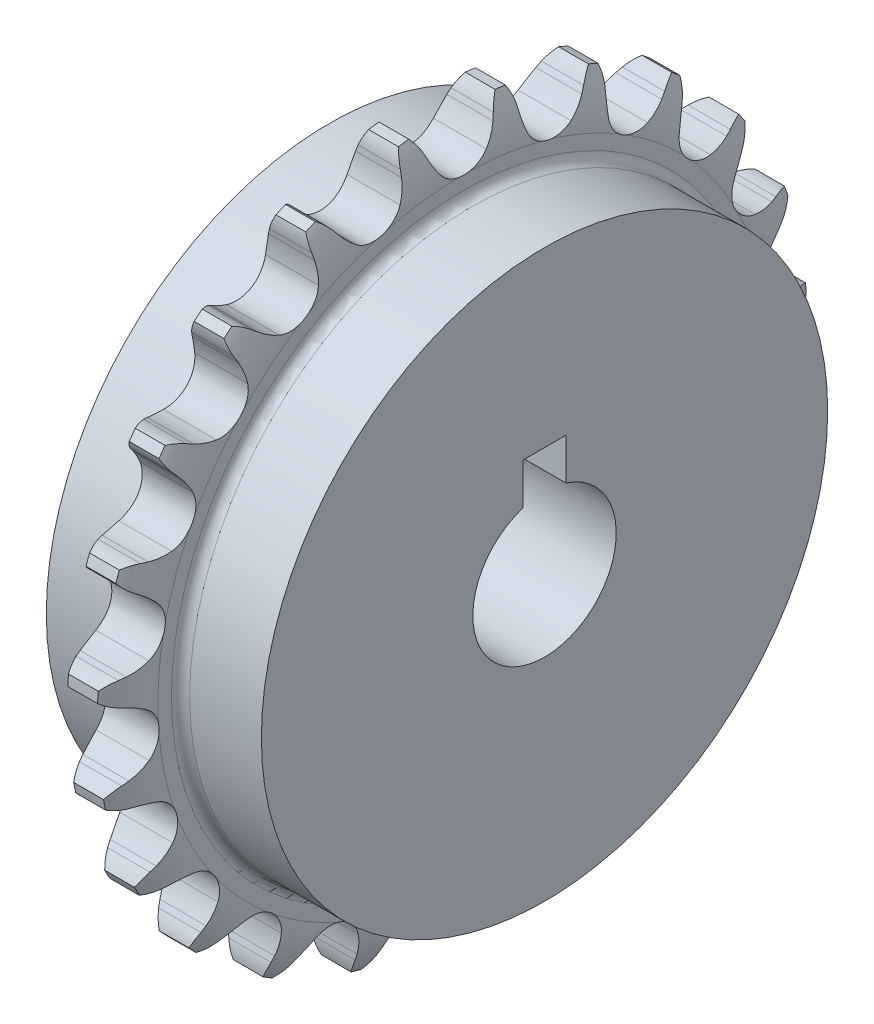
from build123d import *

# Parameters (mm, degrees)
EXTRUDECUTONE_DEPTH      = 5.315766473
PATTERNONE_COUNT         = 23
SKETCH_1_2_R             = 39.5
EXTRUDE_1_DEPTH          = 15
CUT_EXTRUDE_B_DEPTH      = 72.543477978
CUT_EXTRUDE_B_DEPTH_BACK = 72.543477978


with BuildPart() as part:
    # Sketch 1 → Revolve 2 (revolve)
    with BuildSketch(Plane.XY, mode=Mode.PRIVATE) as revolve_2_sk:
        with BuildLine():
            Line((-5.315766473, 0), (-5.315766473, 39.5))
            Line((-5.315766473, 39.5), (-4.998363178, 39.5))
            ThreePointArc((-4.998363178, 39.5), (-4.10061109, 39.87186109), (-3.72875, 40.769613178))
            Line((-3.72875, 40.769613178), (-3.72875, 42.674032945))
            ThreePointArc((-3.72875, 42.674032945), (-3.384453661, 46.203405438), (-2.07775, 49.5))
            Line((-2.07775, 49.5), (2.07775, 49.5))
            ThreePointArc((2.07775, 49.5), (3.384453661, 46.203405438), (3.72875, 42.674032945))
            Line((3.72875, 42.674032945), (3.72875, 40.769613178))
            ThreePointArc((3.72875, 40.769613178), (4.10061109, 39.87186109), (4.998363178, 39.5))
            Line((4.998363178, 39.5), (5.315766473, 39.5))
            Line((5.315766473, 39.5), (5.315766473, 0))
            Line((5.315766473, 0), (-5.315766473, 0))
        make_face()
    revolve(revolve_2_sk.sketch.rotate(Axis((-4, 0, 0), (1, 0, 0)), 90), axis=Axis((-4, 0, 0), (1, 0, 0)))

    # 草图2 → ExtrudeCutOne (cut, symmetric)
    with BuildSketch(Plane(origin=(0, 0, 0), x_dir=(0, 0, -1), z_dir=(1, 0, 0))):
        with BuildLine():
            Line((4.588692581, 46.610285416), (4.899653292, 47.378261808))
            ThreePointArc((4.899653292, 47.378261808), (5.378614734, 48.306828579), (6.018529669, 49.132751812))
            ThreePointArc((6.018529669, 49.132751812), (0, 49.5), (-6.018529669, 49.132751812))
            ThreePointArc((-6.018529669, 49.132751812), (-5.378614734, 48.306828579), (-4.899653292, 47.378261808))
            Line((-4.899653292, 47.378261808), (-4.588692581, 46.610285416))
            ThreePointArc((-4.588692581, 46.610285416), (-3.973376288, 45.345046883), (-3.192395607, 44.174785433))
            ThreePointArc((-3.192395607, 44.174785433), (0, 42.604232945), (3.192395607, 44.174785433))
            ThreePointArc((3.192395607, 44.174785433), (3.973376288, 45.345046883), (4.588692581, 46.610285416))
        make_face()
    extrudecutone = extrude(amount=EXTRUDECUTONE_DEPTH, both=True, mode=Mode.SUBTRACT)

    # PatternOne: ExtrudeCutOne ×23 about axis
    patternone_axis = Axis((0, 0, 0), (1, 0, 0))
    for i in range(1, PATTERNONE_COUNT):
        add(extrudecutone.rotate(patternone_axis, i * 360 / PATTERNONE_COUNT), mode=Mode.SUBTRACT)

    # Sketch 1 2 → 凸台-拉伸1 (add, symmetric)
    with BuildSketch(Plane(origin=(0, 0, 0), x_dir=(0, 0, -1), z_dir=(1, 0, 0))):
        with Locations(Location((0, 0, 0), (0, 0, 180))):
            Circle(SKETCH_1_2_R)
    extrude(amount=EXTRUDE_1_DEPTH, both=True)

    # 草图Key → 切除-拉伸B (cut, two sides: drawn at the far end of the back side and taken through both)
    with BuildSketch(Plane(origin=(0, 0, 0), x_dir=(0, 0, -1), z_dir=(1, 0, 0)).offset(-CUT_EXTRUDE_B_DEPTH_BACK)):
        with BuildLine():
            Line((-3, 9.539392014), (-3, 15.321216067))
            Line((-3, 15.321216067), (3, 15.321216067))
            Line((3, 15.321216067), (3, 9.539392014))
            ThreePointArc((3, 9.539392014), (0, -10), (-3, 9.539392014))
        make_face()
    extrude(amount=CUT_EXTRUDE_B_DEPTH + CUT_EXTRUDE_B_DEPTH_BACK, mode=Mode.SUBTRACT)


solid = part.part
